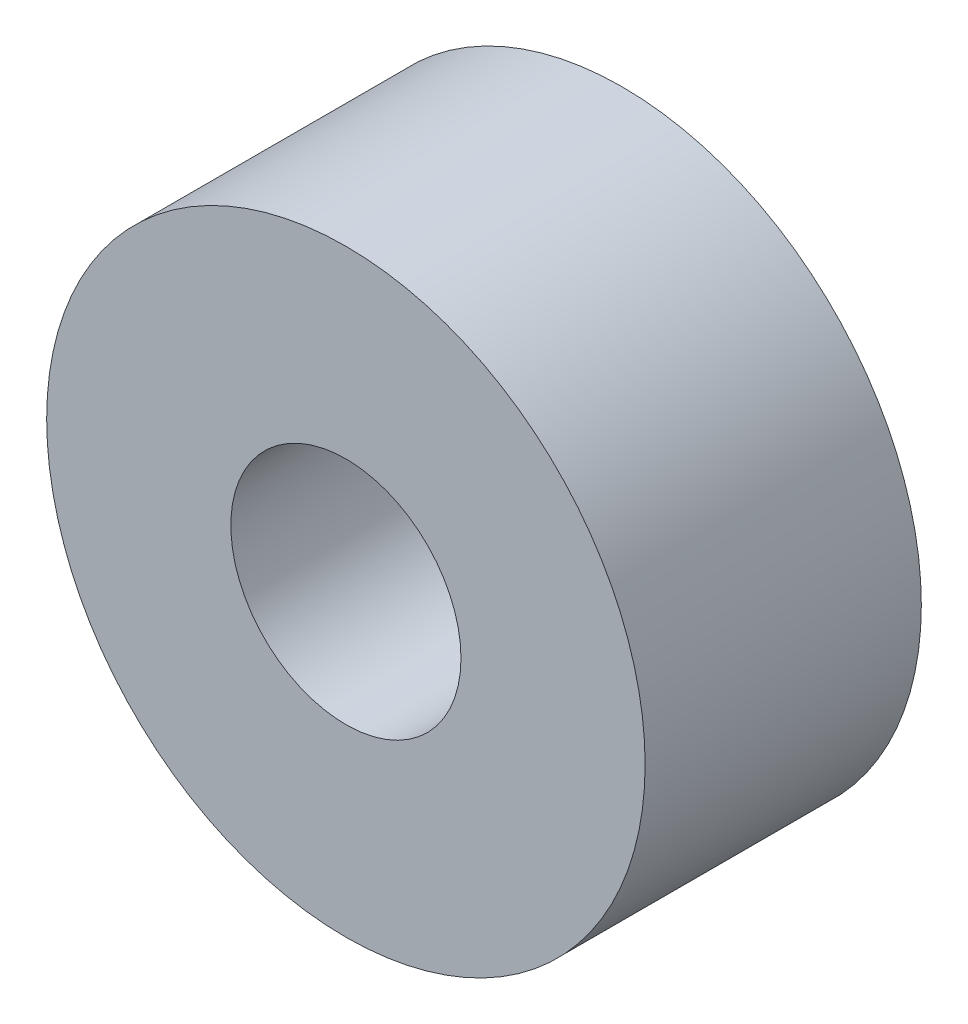
SolidWorks part; units mm, degrees
ref_plane "Front Plane" through (0, 0, 0) normal (0, 0, 1) x (1, 0, 0)
ref_plane "Top Plane" through (0, 0, 0) normal (0, 1, 0) x (1, 0, 0)
ref_plane "Right Plane" through (0, 0, 0) normal (1, 0, 0) x (0, 0, -1)
other "Configuration Table"
sketch "Sketch2" plane through (0, 0, 0) normal (0, 0, 1) x (1, 0, 0)
  circle A1 centre (0, 0) radius 2.5
  circle A2 centre (0, 0) radius 6.5
extrude "Boss-Extrude1" add sketch "Sketch2" along normal blind 6
